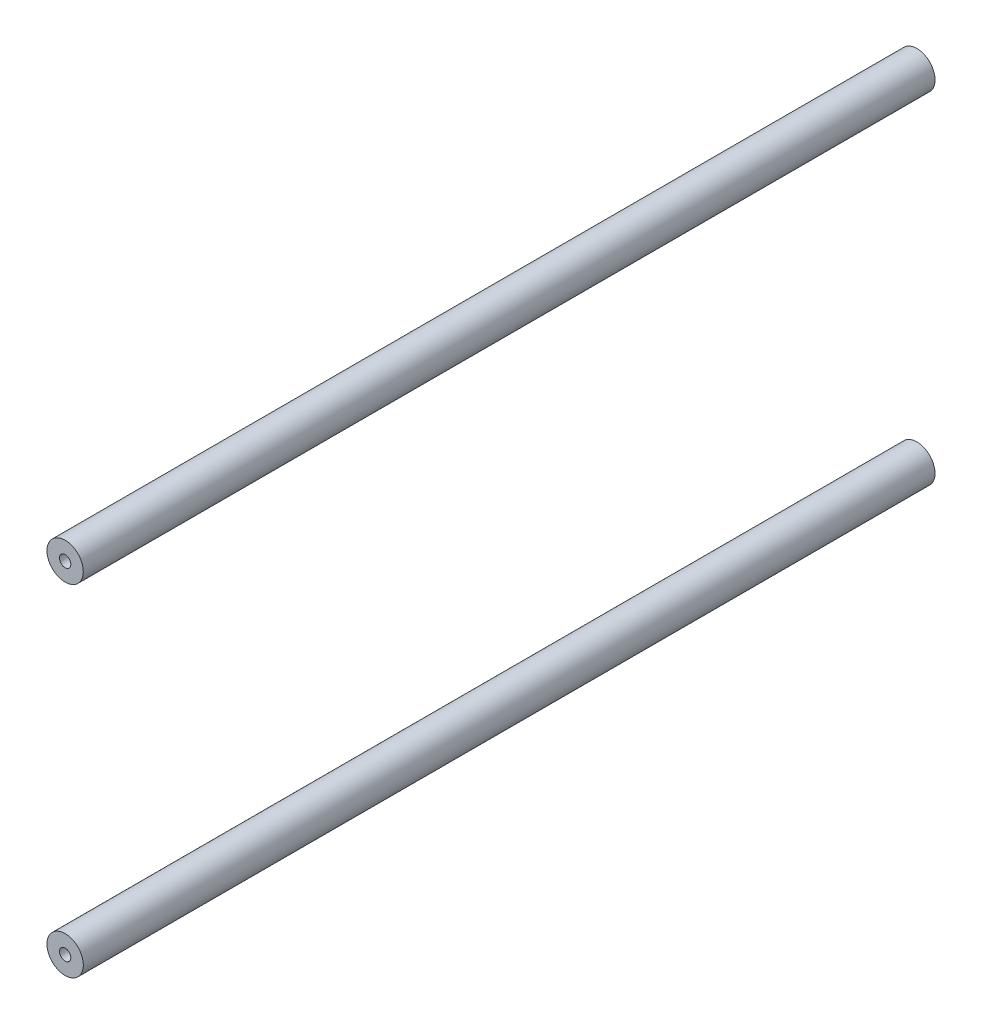
from build123d import *

# Parameters (mm, degrees)
SKETCH1_R                  = 8
BOSS_EXTRUDE1_DEPTH        = 375
BOSS_EXTRUDE1_2_DEPTH      = 375
SKETCH3_W                  = 2.5
SKETCH3_H                  = 375
M6_TAPPED_HOLE1_AT_2_COUNT = 2
M6_TAPPED_HOLE1_AT_2_PITCH = 150


with BuildPart() as part:
    # Sketch1 → Boss-Extrude1 (new body)
    with BuildSketch(Plane.XY):
        with Locations((-78, 75)):
            Circle(SKETCH1_R)
    extrude(amount=BOSS_EXTRUDE1_DEPTH)

    # Sketch3 → M6 Tapped Hole1 (revolve, cut)
    with BuildSketch(Plane(origin=(-78, 75, 0), x_dir=(0, 1, 0), z_dir=(1, 0, 0))):
        with Locations((1.25, 187.5)):
            Rectangle(SKETCH3_W, SKETCH3_H)
    m6_tapped_hole1 = revolve(axis=Axis((-78, 75, -6.35), (0, 0, 1)), mode=Mode.SUBTRACT)


with BuildPart() as body_2:
    # Sketch1 → Boss-Extrude1 2 (new body)
    with BuildSketch(Plane.XY):
        with Locations(Location((-78, -75, 0), (0, 0, 180))):
            Circle(SKETCH1_R)
    extrude(amount=BOSS_EXTRUDE1_2_DEPTH)

    # M6 Tapped Hole1 at 2: M6 Tapped Hole1 ×2
    with Locations(*[(0, -i * M6_TAPPED_HOLE1_AT_2_PITCH, 0) for i in range(1, M6_TAPPED_HOLE1_AT_2_COUNT)]):
        add(m6_tapped_hole1, mode=Mode.SUBTRACT)


solid = Compound([part.part, body_2.part])
